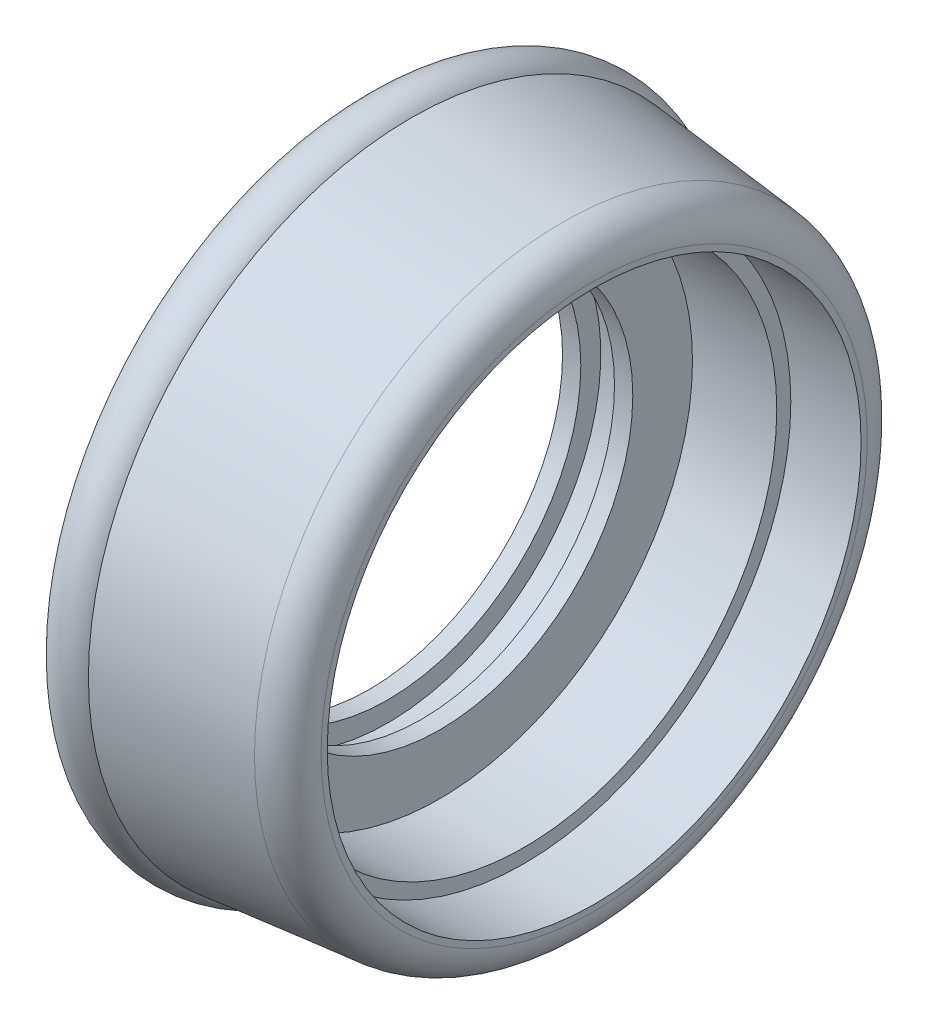
from build123d import *


with BuildPart() as part:
    # Sketch1 → Revolve1 (revolve)
    with BuildSketch(Plane.XY, mode=Mode.PRIVATE) as revolve1_sk:
        with BuildLine():
            Line((0, 27.5), (0, 46))
            ThreePointArc((0, 46), (3, 47.354248689), (6, 46))
            Line((6, 46), (27.497518595, 43.85024814))
            ThreePointArc((27.497518595, 43.85024814), (30.707262668, 42.230088793), (32, 38.875062189))
            Line((32, 38.875062189), (32, 38))
            Line((32, 38), (22, 38))
            Line((22, 38), (22, 36))
            Line((22, 36), (10, 36))
            Line((10, 36), (10, 27.5))
            Line((10, 27.5), (7.4, 27.5))
            Line((7.4, 27.5), (7.4, 30.35))
            Line((7.4, 30.35), (2.6, 30.35))
            Line((2.6, 30.35), (2.6, 27.5))
            Line((2.6, 27.5), (0, 27.5))
        make_face()
    revolve(revolve1_sk.sketch.rotate(Axis((-44.681900546, 0, 0), (1, 0, 0)), 90), axis=Axis((-44.681900546, 0, 0), (1, 0, 0)))


solid = part.part
